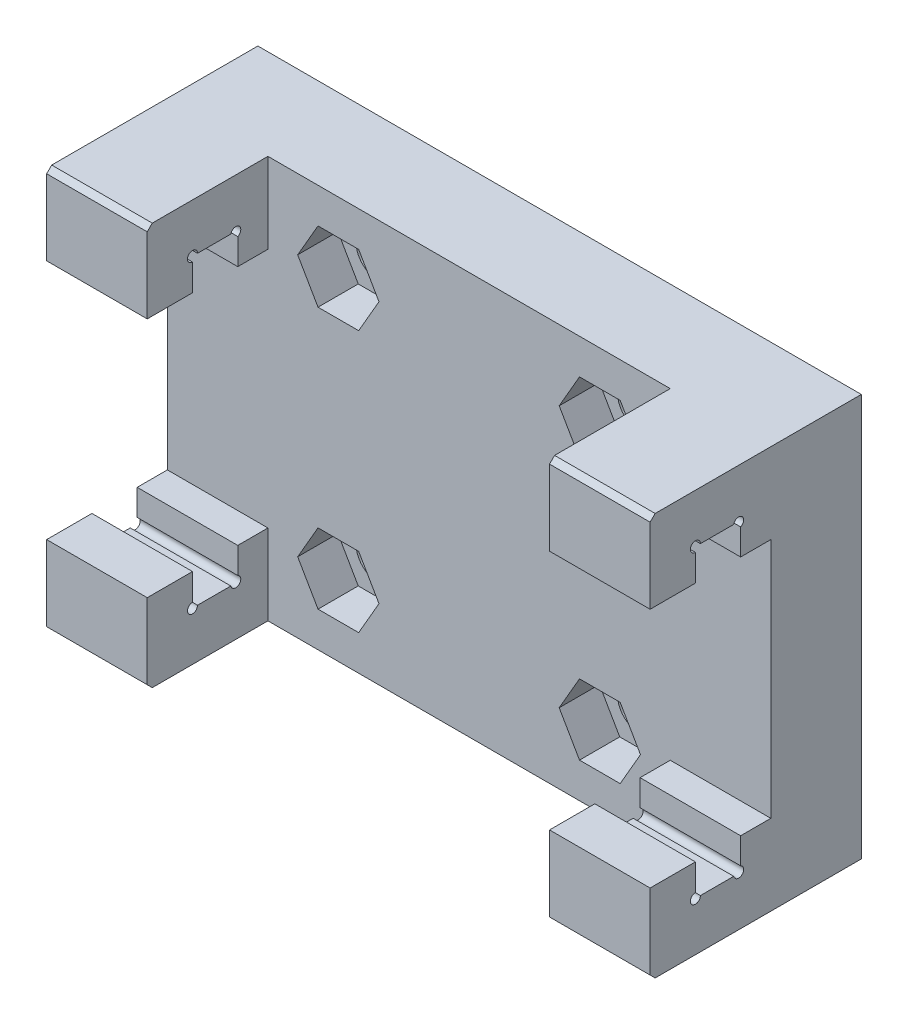
SolidWorks part; units mm, degrees
ref_plane "前视基准面" through (0, 0, 0) normal (0, 0, 1) x (1, 0, 0)
ref_plane "上视基准面" through (0, 0, 0) normal (0, 1, 0) x (1, 0, 0)
ref_plane "右视基准面" through (0, 0, 0) normal (1, 0, 0) x (0, 0, -1)
sketch "草图1" plane through (0, 0, 0) normal (0, 0, 1) x (1, 0, 0)
  line L1 (-30, 20) -> (30, 20)
  line L2 (-30, 20) -> (-30, -20)
  line L3 (-30, -20) -> (30, -20)
  line L4 (30, 20) -> (30, -20)
  line L5 (-30, 20) -> (30, -20) construction
  line L6 (-30, -20) -> (30, 20) construction
  point P0 (0, 0)
  dimension "D1" = 60
  dimension "D2" = 40
extrude "凸台-拉伸1" add sketch "草图1" along normal blind 21
sketch "草图2" plane through (0, 0, 21) normal (0, 0, 1) x (1, 0, 0)
  line L1 (-20, 23.0564) -> (20, 23.0564)
  line L2 (-20, 23.0564) -> (-20, -23.0564)
  line L3 (-20, -23.0564) -> (20, -23.0564)
  line L4 (20, 23.0564) -> (20, -23.0564)
  line L5 (-20, 23.0564) -> (20, -23.0564) construction
  line L6 (-20, -23.0564) -> (20, 23.0564) construction
  point P0 (0, 0)
  dimension "D1" = 40
extrude "切除-拉伸1" cut sketch "草图2" against normal blind 12
sketch "草图3" plane through (0, 0, 21) normal (0, 0, 1) x (1, 0, 0)
  line L1 (-40.2568, 12) -> (40.2568, 12)
  line L2 (-40.2568, 12) -> (-40.2568, -12)
  line L3 (-40.2568, -12) -> (40.2568, -12)
  line L4 (40.2568, 12) -> (40.2568, -12)
  line L5 (-40.2568, 12) -> (40.2568, -12) construction
  line L6 (-40.2568, -12) -> (40.2568, 12) construction
  point P0 (0, 0)
  dimension "D1" = 24
extrude "切除-拉伸2" cut sketch "草图3" against normal blind 12
sketch "草图4" plane through (-30, 0, 0) normal (-1, 0, 0) x (0, 0, 1)
  line L0 (21, 20) -> (21, 12) construction
  line L1 (12, 15.15) -> (16.5, 15.15)
  line L2 (12, 15.15) -> (12, -15.15)
  line L3 (12, -15.15) -> (16.5, -15.15)
  line L4 (16.5, 15.15) -> (16.5, -15.15)
  dimension "D1" = 30.3
  dimension "D2" = 4.5
  dimension "D3" = 4.5
  dimension "D4" = 15.15
extrude "切除-拉伸3" cut sketch "草图4" against normal through all
sketch "草图5" plane through (0, 0, 9) normal (0, 0, 1) x (1, 0, 0)
  circle A0 centre (-13, 13) radius 2.25
  dimension "D2" = 13
  dimension "D3" = 4.5
  dimension "D1" = 13
extrude "切除-拉伸4" cut sketch "草图5" against normal blind 12
mirror "镜向1" about plane through (0, 0, 0) normal (0, 1, 0) of "切除-拉伸4"
mirror "镜向2" about plane through (0, 0, 0) normal (1, 0, 0) of "镜向1", "切除-拉伸4"
sketch "草图6" plane through (0, 0, 9) normal (0, 0, 1) x (1, 0, 0)
  line L1 (-8.9585, 13) -> (-10.9793, 16.5)
  line L2 (-10.9793, 16.5) -> (-15.0207, 16.5)
  line L3 (-15.0207, 16.5) -> (-17.0415, 13)
  line L4 (-17.0415, 13) -> (-15.0207, 9.5)
  line L5 (-15.0207, 9.5) -> (-10.9793, 9.5)
  line L6 (-10.9793, 9.5) -> (-8.9585, 13)
  circle A0 centre (-13, 13) radius 3.5 construction
extrude "切除-拉伸5" cut sketch "草图6" against normal blind 4
mirror "镜向3" about plane through (0, 0, 0) normal (1, 0, 0) of "切除-拉伸5"
mirror "镜向4" about plane through (0, 0, 0) normal (0, 1, 0) of "镜向3", "切除-拉伸5"
sketch "草图7" plane through (-30, 0, 0) normal (-1, 0, 0) x (0, 0, 1)
  circle A0 centre (12.2, 15.05) radius 0.5
  circle A1 centre (16.5, 15.15) radius 0.5
extrude "切除-拉伸6" cut sketch "草图7" against normal through all
mirror "镜向5" about plane through (0, 0, 0) normal (0, 1, 0) of "切除-拉伸6"
chamfer "倒角1" distance 0.5 angle 45 4 edges at (25, -20, 21) (-25, -20, 21) (25, 20, 21) (-25, 20, 21)
